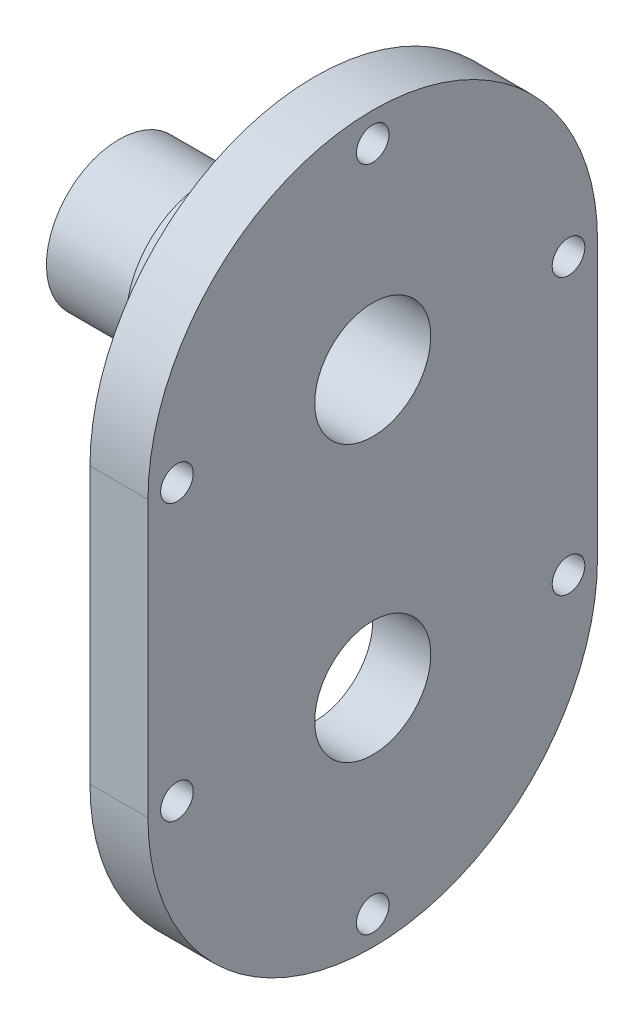
SolidWorks part; units mm, degrees
ref_plane "Front Plane" through (0, 0, 0) normal (0, 0, 1) x (1, 0, 0)
ref_plane "Top Plane" through (0, 0, 0) normal (0, 1, 0) x (1, 0, 0)
ref_plane "Right Plane" through (0, 0, 0) normal (1, 0, 0) x (0, 0, -1)
other "Configuration Table"
ref_plane "Plane1" through (8, 0, 0) normal (1, 0, 0) x (0, 0, -1)
sketch "Sketch1" plane through (8, 0, 0) normal (1, 0, 0) x (0, 0, -1)
  line L0 (31, -19) -> (31, 19)
  line L1 (-31, 19) -> (-31, -19)
  arc A0 (-31, -19) -> (31, -19) centre (0, -19) ccw
  arc A1 (31, 19) -> (-31, 19) centre (0, 19) ccw
extrude "Boss-Extrude1" add sketch "Sketch1" against normal blind 8
sketch "Sketch2" plane through (0, 0, 0) normal (0, 0, 1) x (1, 0, 0)
  line L0 (-27, 29) -> (-27, 19)
  line L1 (-27, 19) -> (0, 19)
  line L2 (0, 19) -> (0, 30.7861)
  line L3 (0, 30.7861) -> (-15, 30)
  line L4 (-15, 30) -> (-15, 29)
  line L5 (-15, 29) -> (-27, 29)
  line L6 (-27, 19) -> (0, 19) construction
revolve "Revolve1" add sketch "Sketch2" angle 360 about L6
hole_wizard "Ø16.0 (16) Diameter Hole1" positions "Sketch4" profile "Sketch3" hole size "Ø16.0" standard "ANSI Metric"
sketch "Sketch4" plane through (0, 0, 0) normal (-1, 0, 0) x (0, 0, 1)
  point P0 (0, -19)
sketch "Sketch3" plane through (0, -19, 0) normal (0, 1, 0) x (0, 0, 1)
  line L0 (0, 0) -> (0, 8)
  line L1 (0, 8) -> (8, 8)
  line L2 (8, 8) -> (8, 0)
  line L5 (8, 0) -> (0, 0)
  line L11 (0, -6.35) -> (0, 107.95) construction
  dimension "通孔孔直径" = 16
  dimension "通孔孔深度" = 8
hole_wizard "Ø16.0 (16) Diameter Hole2" positions "Sketch6" profile "Sketch5" hole size "Ø16.0" standard "ANSI Metric"
sketch "Sketch6" plane through (-27, 0, 0) normal (-1, 0, 0) x (0, 0, 1)
  point P0 (0, 19)
sketch "Sketch5" plane through (-27, 19, 0) normal (0, 1, 0) x (0, 0, 1)
  line L0 (0, 0) -> (0, 35)
  line L1 (0, 35) -> (8, 35)
  line L2 (8, 35) -> (8, 1.8)
  line L3 (8, 1.8) -> (9.8, 0)
  line L5 (9.8, 0) -> (0, 0)
  line L6 (-8, 1.8) -> (-9.8, 0) construction
  line L11 (0, -6.35) -> (0, 107.95) construction
  dimension "通孔孔直径" = 16
  dimension "通孔孔深度" = 35
  dimension "近端锥形沉头孔直径" = 19.6
  dimension "近端锥形沉头孔角度" = 90
hole_wizard "Ø4.5 (4.5) Diameter Hole1" positions "Sketch8" profile "Sketch7" hole size "Ø4.5" standard "ANSI Metric"
sketch "Sketch8" plane through (0, 0, 0) normal (-1, 0, 0) x (0, 0, 1)
  point P0 (0, 46)
  point P1 (27, 19)
  point P2 (-27, 19)
  point P3 (27, -19)
  point P4 (-27, -19)
  point P5 (0, -46)
sketch "Sketch7" plane through (0, 46, 0) normal (0, 1, 0) x (0, 0, 1)
  line L0 (0, 0) -> (0, 8)
  line L1 (0, 8) -> (2.25, 8)
  line L2 (2.25, 8) -> (2.25, 0)
  line L5 (2.25, 0) -> (0, 0)
  line L11 (0, -6.35) -> (0, 107.95) construction
  dimension "通孔孔直径" = 4.5
  dimension "通孔孔深度" = 8
chamfer "Chamfer1" distance 1.5 angle 45 6 edges at (0, 19, 29.25) (0, 46, 2.25) (0, 19, -24.75) (0, -19, -24.75) (0, -46, 2.25) (0, -19, 29.25)
